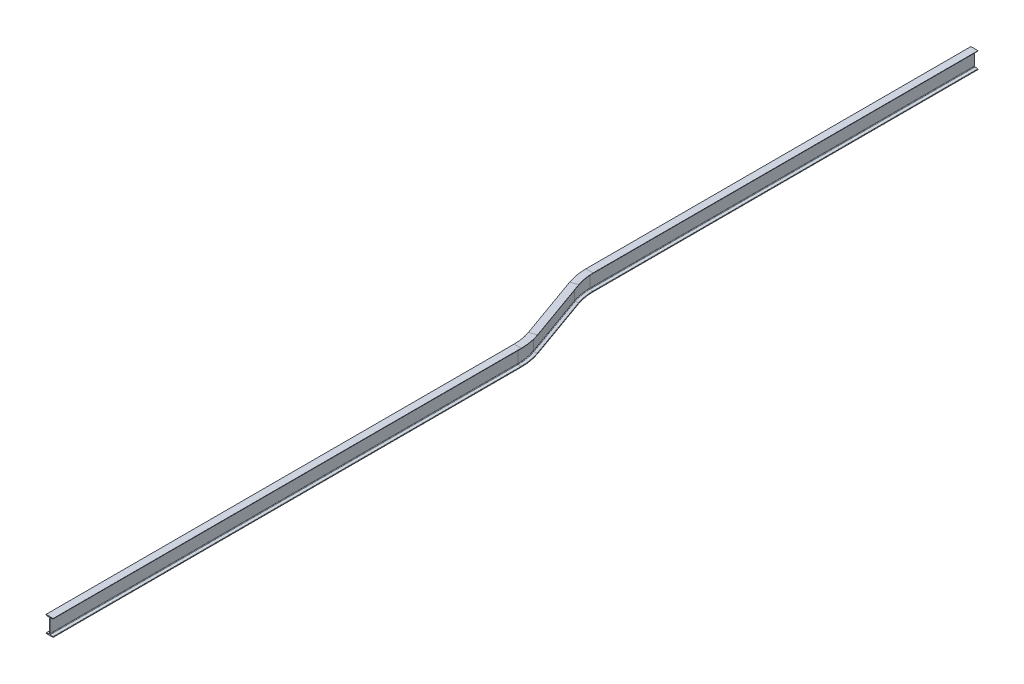
from build123d import *


with BuildPart() as part:
    # Sweep1: sweep along a path in Sketch2
    with BuildLine(Plane(origin=(0, 0, 0), x_dir=(1, 0, 0), z_dir=(0, 1, 0))) as sweep1_path:
        Line((0, 0), (0, 7989.288529227))
        ThreePointArc((0, 7989.288529227), (-13.773697715, 8149.615809986), (-54.691142459, 8305.244581169))
        Line((-54.691142459, 8305.244581169), (-445.308857541, 9399.755418831))
        ThreePointArc((-445.308857541, 9399.755418831), (-486.226302285, 9555.384190014), (-500, 9715.711470773))
        Line((-500, 9715.711470773), (-500, 16285))
    # Sketch1 → Sweep1 (sweep)
    with BuildSketch(Plane.XY):
        with BuildLine():
            Line((-61, 280), (-61, 276.227273568))
            ThreePointArc((-61, 276.227273568), (-59.744005907, 272.801486619), (-56.571314633, 270.999385772))
            Line((-56.571314633, 270.999385772), (-13.023810633, 263.741468439))
            ThreePointArc((-13.023810633, 263.741468439), (-6.738290184, 260.171268648), (-4.25, 253.384332239))
            Line((-4.25, 253.384332239), (-4.25, 26.615667761))
            ThreePointArc((-4.25, 26.615667761), (-6.738290184, 19.828731352), (-13.023810633, 16.258531561))
            Line((-13.023810633, 16.258531561), (-56.571314633, 9.000614228))
            ThreePointArc((-56.571314633, 9.000614228), (-59.744005907, 7.198513381), (-61, 3.772726432))
            Line((-61, 3.772726432), (-61, 0))
            Line((-61, 0), (61, 0))
            Line((61, 0), (61, 3.772726432))
            ThreePointArc((61, 3.772726432), (59.744005907, 7.198513381), (56.571314633, 9.000614228))
            Line((56.571314633, 9.000614228), (13.023810633, 16.258531561))
            ThreePointArc((13.023810633, 16.258531561), (6.738290184, 19.828731352), (4.25, 26.615667761))
            Line((4.25, 26.615667761), (4.25, 253.384332239))
            ThreePointArc((4.25, 253.384332239), (6.738290184, 260.171268648), (13.023810633, 263.741468439))
            Line((13.023810633, 263.741468439), (56.571314633, 270.999385772))
            ThreePointArc((56.571314633, 270.999385772), (59.744005907, 272.801486619), (61, 276.227273568))
            Line((61, 276.227273568), (61, 280))
            Line((61, 280), (-61, 280))
        make_face()
    sweep(path=sweep1_path.line)


solid = part.part
